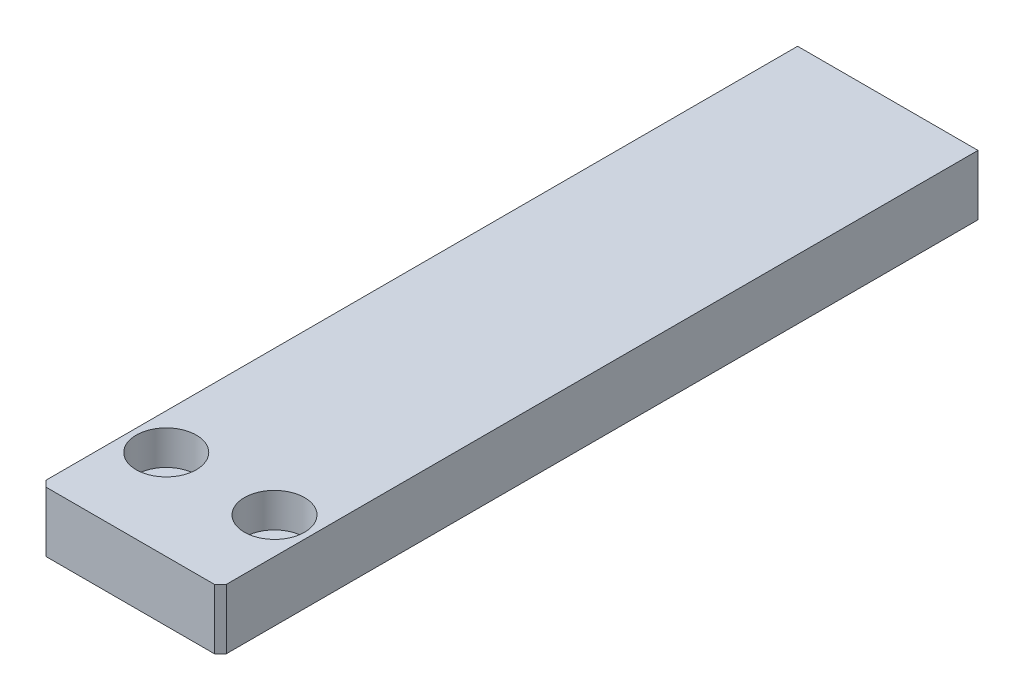
SolidWorks part; units mm, degrees
material "A6061"
ref_plane "前基準面" through (0, 0, 0) normal (0, 0, 1) x (1, 0, 0)
ref_plane "上基準面" through (0, 0, 0) normal (0, 1, 0) x (1, 0, 0)
ref_plane "右基準面" through (0, 0, 0) normal (1, 0, 0) x (0, 0, -1)
sketch "草图1" plane through (0, 0, 0) normal (0, 1, 0) x (1, 0, 0)
  line L1 (-15, -63) -> (15, -63)
  line L2 (-15, -63) -> (-15, 63)
  line L3 (-15, 63) -> (15, 63)
  line L4 (15, -63) -> (15, 63)
  line L5 (-15, -63) -> (15, 63) construction
  line L6 (-15, 63) -> (15, -63) construction
  point P0 (0, 0)
  dimension "D1" = 30
  dimension "D2" = 126
extrude "凸台-拉伸1" add sketch "草图1" along normal mid plane 10
hole_wizard "打孔尺寸(%根据)内六角圆柱头螺钉的类型1" positions "草图2" profile "草图3" counterbore size "M5" standard "GB" end condition through all
sketch "草图2" plane through (0, 5, 0) normal (0, 1, 0) x (1, 0, 0)
  line L0 (0, -40.7311) -> (0, 0) construction
  line L2 (-15, -63) -> (15, -63) construction
  point P0 (9, -48)
  point P11 (-9, -48)
  dimension "D1" = 18
  dimension "D3" = 15
sketch "草图3" plane through (9, 5, 48) normal (1, 0, 0) x (0, 0, 1)
  line L0 (0, 0) -> (0, 10)
  line L1 (0, 10) -> (2.75, 10)
  line L3 (2.75, 10) -> (2.75, 5.7)
  line L4 (2.75, 5.7) -> (5, 5.7)
  line L5 (5, 5.7) -> (5, 0)
  line L7 (5, 0) -> (0, 0)
  line L11 (0, -6.35) -> (0, 107.95) construction
  dimension "通孔孔直径" = 5.5
  dimension "通孔孔深度" = 10
  dimension "柱形沉头孔直径" = 10
  dimension "柱形沉头孔深度" = 5.7
chamfer "倒角1" distance 1 angle 45 2 edges at (15, 0, 63) (-15, 0, 63)
hole_wizard "M4 螺纹孔1" positions "草图4" profile "草图5" tap size "M4" standard "GB"
sketch "草图4" plane through (0, 0, -63) normal (0, 0, -1) x (-1, 0, 0)
  line L0 (0, 10.6516) -> (0, 0) construction
  point P0 (-10, 0)
  point P6 (10, 0)
  dimension "D1" = 20
sketch "草图5" plane through (10, 0, -63) normal (1, 0, 0) x (0, 1, 0)
  line L0 (0, 0) -> (0, 11.0914)
  line L1 (0, 11.0914) -> (1.65, 10.1)
  line L2 (1.65, 10.1) -> (1.65, 0)
  line L5 (1.65, 0) -> (0, 0)
  line L10 (0, 11.0914) -> (-1.65, 10.1) construction
  line L11 (0, -6.35) -> (0, 107.95) construction
  dimension "螺纹孔钻头直径" = 3.3
  dimension "螺纹孔钻头深度" = 10.1
  dimension "导头角度" = 118
cosmetic thread "孔螺蚊线1" parameters "D1"=8, "D2"=4
cosmetic thread "孔螺蚊线2" parameters "D1"=8, "D2"=4
